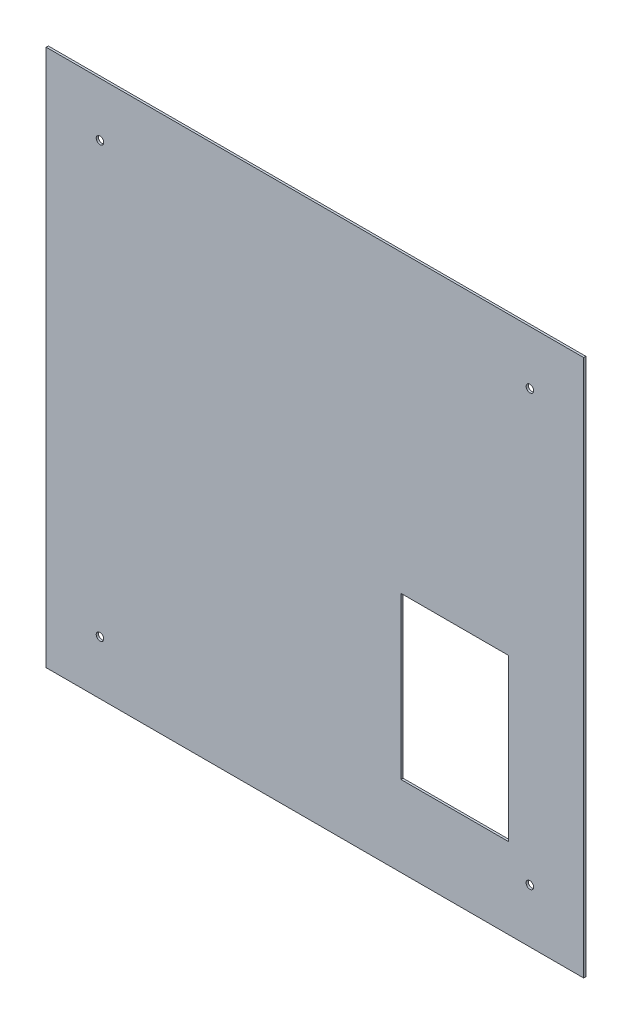
from build123d import *

# Parameters (mm, degrees)
SKETCH_1_W            = 500
SKETCH_1_H            = 500
EXTRUDE_1_DEPTH       = 2
HOLE_WIZARD_7_0_7_1_D = 7
SKETCH_4_W            = 100
SKETCH_4_H            = 150
CUT_EXTRUDE_1_DEPTH   = 354.559047402


with BuildPart() as part:
    # 草图1 → 凸台-拉伸1 (new body)
    with BuildSketch(Plane.XY):
        Rectangle(SKETCH_1_W, SKETCH_1_H)
    extrude(amount=EXTRUDE_1_DEPTH)

    # Ø7.0 (7) 直径孔1 (through all)
    with Locations(Plane.XY.offset(2)):
        with Locations((-200, 200), (200, 200), (-200, -200), (200, -200)):
            Hole(HOLE_WIZARD_7_0_7_1_D / 2)

    # 草图4 → 切除-拉伸1 (cut, through all)
    with BuildSketch(Plane.XY.offset(2)):
        with Locations((130, -100)):
            Rectangle(SKETCH_4_W, SKETCH_4_H)
    extrude(amount=-CUT_EXTRUDE_1_DEPTH, mode=Mode.SUBTRACT)


solid = part.part
